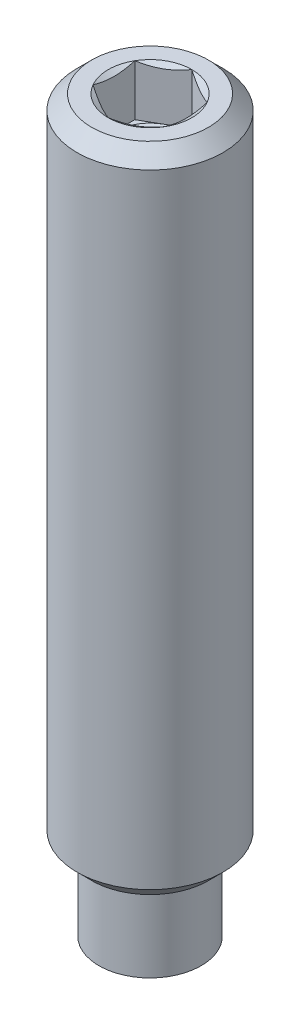
from build123d import *

# Parameters (mm, degrees)
SKETCH1_R           = 5
BOSS_EXTRUDE1_DEPTH = 15
BOSS_EXTRUDE2_START = 35
SKETCH2_R           = 5
BOSS_EXTRUDE2_DEPTH = 35
CUT_EXTRUDE1_DEPTH  = 3.5
SKETCH5_R           = 5
SKETCH5_R_2         = 3.5
CUT_EXTRUDE2_DEPTH  = 5.3
CHAMFER1_SIZE       = 1


with BuildPart() as part:
    # Sketch1 → Boss-Extrude1 (new body)
    with BuildSketch(Plane(origin=(0, 0, 0), x_dir=(1, 0, 0), z_dir=(0, 1, 0))):
        with Locations(Location((0, 0, 0), (0, 0, 270))):
            Circle(SKETCH1_R)
    extrude(amount=BOSS_EXTRUDE1_DEPTH)

    # Sketch2 → Boss-Extrude2 (add)
    with BuildSketch(Plane.XZ.offset(BOSS_EXTRUDE2_START)):
        with Locations(Location((0, 0, 0), (0, 0, 270))):
            Circle(SKETCH2_R)
    extrude(amount=-BOSS_EXTRUDE2_DEPTH)

    # Sketch3 → Cut-Extrude1 (cut)
    with BuildSketch(Plane(origin=(0, 15, 0), x_dir=(1, 0, 0), z_dir=(0, 1, 0))):
        Polygon((0, 2.8615), (-2.478131693, 1.43075), (-2.478131693, -1.43075), (0, -2.8615), (2.478131693, -1.43075), (2.478131693, 1.43075), align=None)
    extrude(amount=-CUT_EXTRUDE1_DEPTH, mode=Mode.SUBTRACT)

    # Sketch4 → Cut-Revolve1 (revolve, cut)
    with BuildSketch(Plane.XY, mode=Mode.PRIVATE) as cut_revolve1_sk:
        Polygon((0, 11.5), (2.478131693, 11.5), (0, 10.06925), align=None)
        Polygon((2.478131693, 14.778662205), (2.478131693, 15), (2.8615, 15), align=None)
    revolve(cut_revolve1_sk.sketch.rotate(Axis((0, -3.932195077, 0), (0, 1, 0)), 90), axis=Axis((0, -3.932195077, 0), (0, 1, 0)), mode=Mode.SUBTRACT)

    # Sketch5 → Cut-Extrude2 (cut)
    with BuildSketch(Plane.XZ.offset(35)):
        with Locations(Location((0, 0, 0), (0, 0, 270))):
            Circle(SKETCH5_R)
        with Locations(Location((0, 0, 0), (0, 0, 270))):
            Circle(SKETCH5_R_2, mode=Mode.SUBTRACT)
    extrude(amount=-CUT_EXTRUDE2_DEPTH, mode=Mode.SUBTRACT)

    # Chamfer1
    chamfer1_edges = [part.edges().sort_by_distance(p)[0] for p in [
        (0, 15, -5),
        (0, -29.7, 5),
    ]]
    chamfer(chamfer1_edges, length=CHAMFER1_SIZE)


solid = part.part
